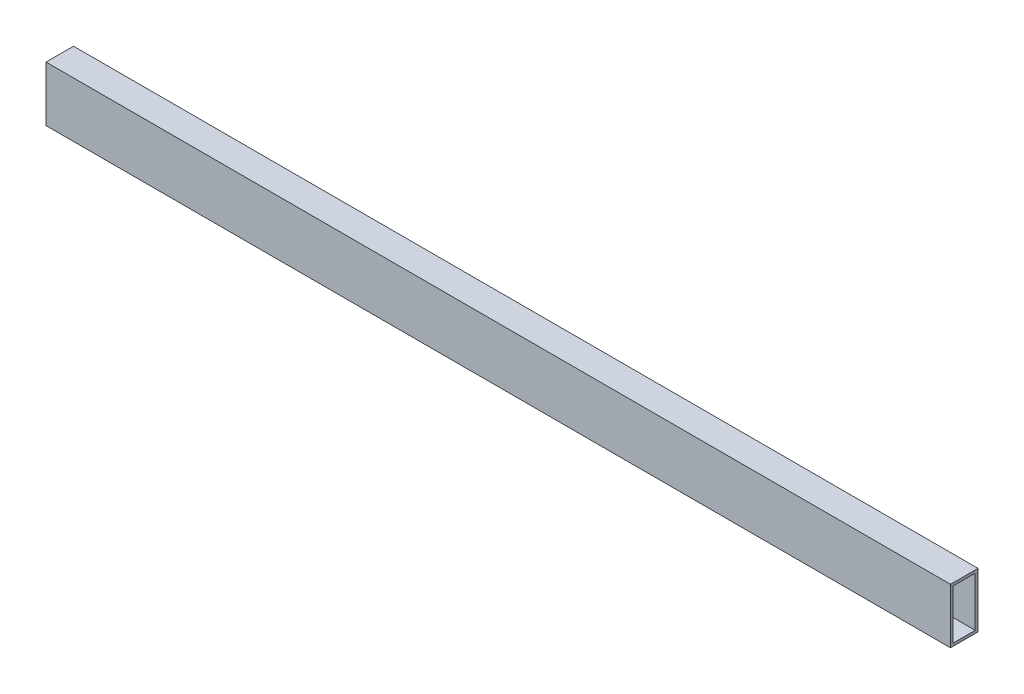
from build123d import *

# Parameters (mm, degrees)
SKETCH1_W           = 986
SKETCH1_H           = 60
BOSS_EXTRUDE1_DEPTH = 30
SKETCH2_W           = 24
SKETCH2_H           = 54
CUT_EXTRUDE1_DEPTH  = 2043


with BuildPart() as part:
    # Sketch1 → Boss-Extrude1 (new body)
    with BuildSketch(Plane.XY):
        Rectangle(SKETCH1_W, SKETCH1_H)
    extrude(amount=BOSS_EXTRUDE1_DEPTH)

    # Sketch2 → Cut-Extrude1 (cut)
    with BuildSketch(Plane.ZY.offset(493)):
        with Locations((15, 0)):
            Rectangle(SKETCH2_W, SKETCH2_H)
    extrude(amount=-CUT_EXTRUDE1_DEPTH, mode=Mode.SUBTRACT)


solid = part.part
